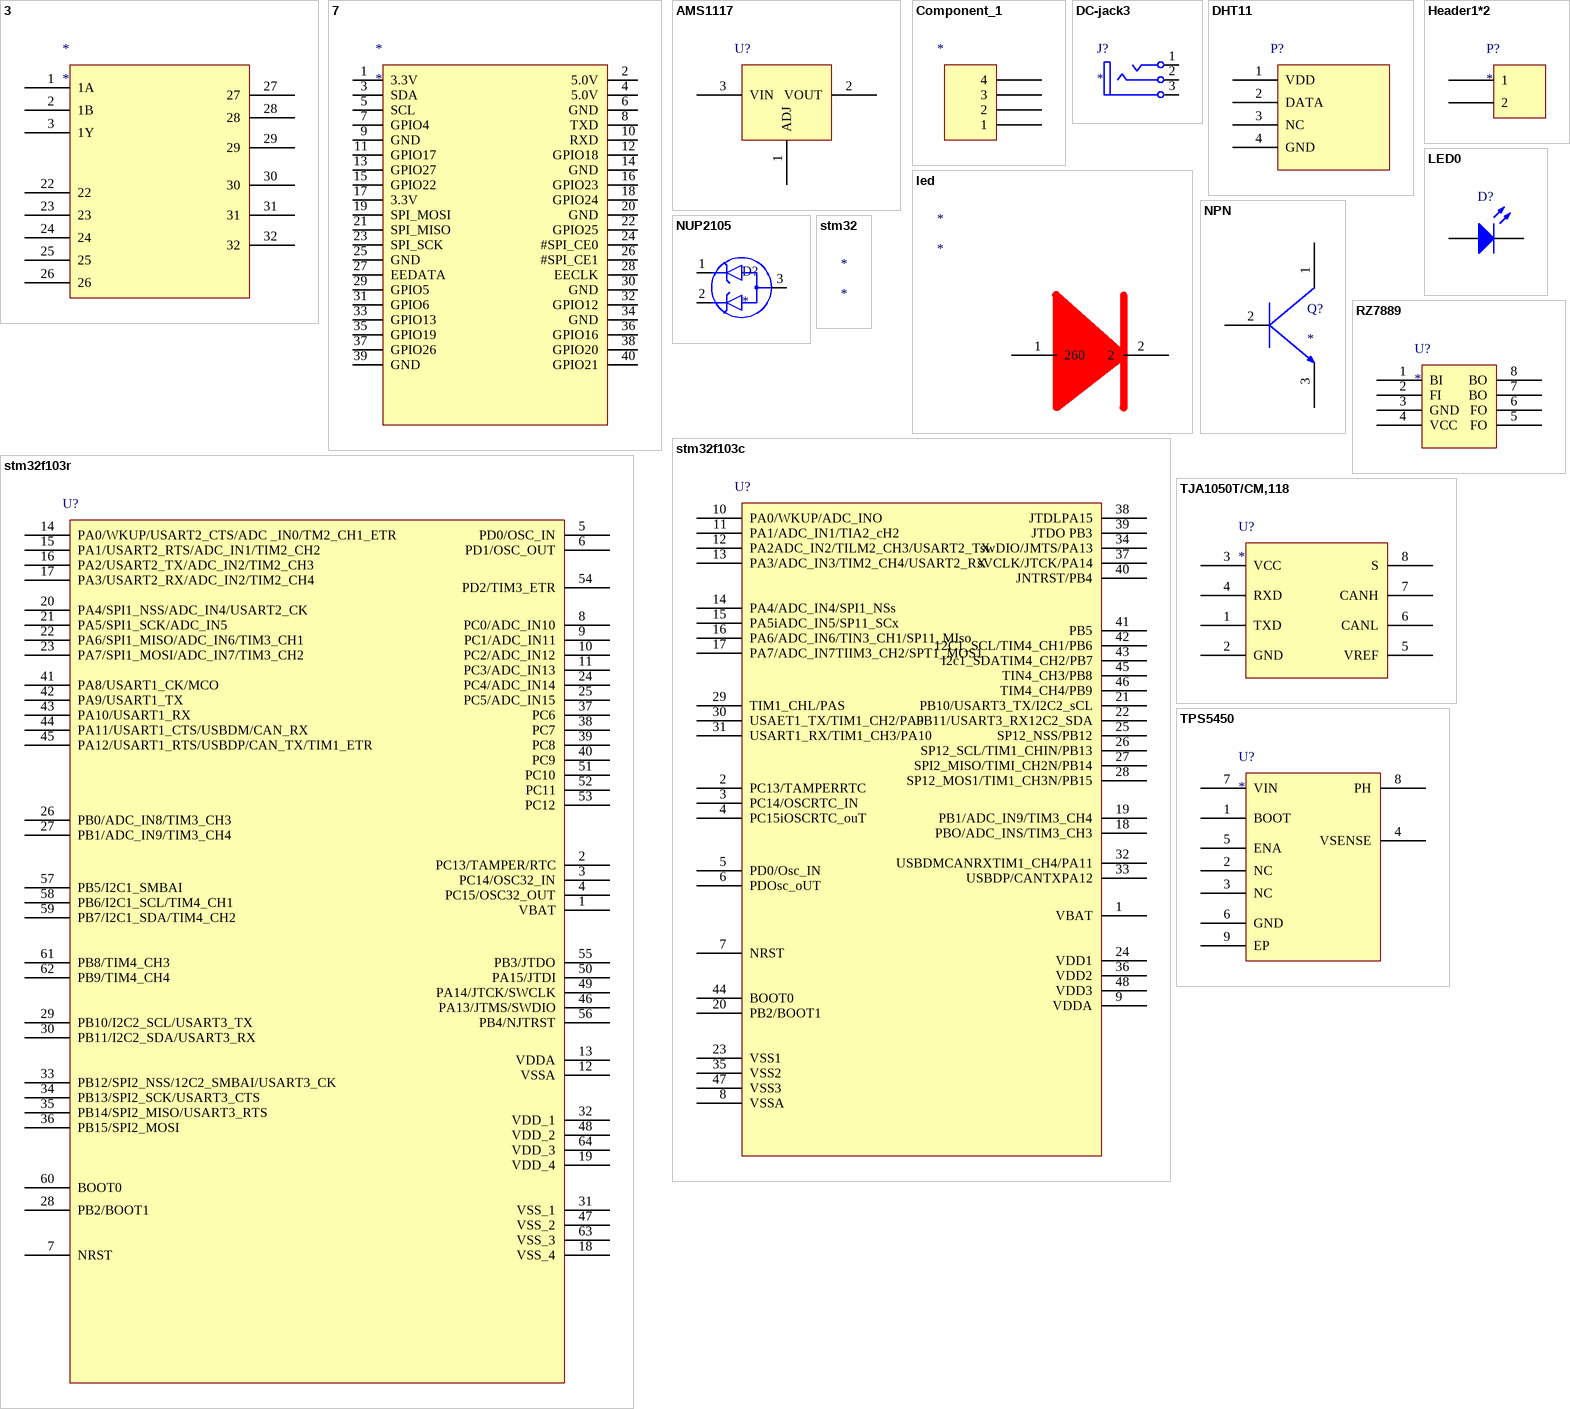
[diagram p0: symbols 3 to TPS5450]
# Altium schematic symbol library MISC82341-24.SchLib: 17 symbols
Pins are listed as number, name and electrical type; pins without a type are passive.


## 3
designator *
pins: 1 1A, 2 1B, 3 1Y, 22, 23, 24, 25, 26, 27, 28, 29, 30, 31, 32

## 7
designator *
pins: 1 3.3V, 2 5.0V, 3 SDA, 4 5.0V, 5 SCL, 6 GND, 7 GPIO4, 8 TXD, 9 GND, 10 RXD, 11 GPIO17, 12 GPIO18, 13 GPIO27, 14 GND, 15 GPIO22, 16 GPIO23, 17 3.3V, 18 GPIO24, 19 SPI_MOSI, 20 GND, 21 SPI_MISO, 22 GPIO25, 23 SPI_SCK, 24 #SPI_CE0, 25 GND, 26 #SPI_CE1, 27 EEDATA, 28 EECLK, 29 GPIO5, 30 GND, 31 GPIO6, 32 GPIO12, 33 GPIO13, 34 GND, 35 GPIO19, 36 GPIO16, 37 GPIO26, 38 GPIO20, 39 GND, 40 GPIO21

## AMS1117
designator U?
footprint SOT-89
pins: 1 ADJ, 2 VOUT, 3 VIN

## Component_1
designator *
pins: ?1 4, ?2 3, ?3 2, ?4 1

## DC-jack3
designator J?
footprint JACK/6-V3
pins: 1 T "Tip/Left Channel/(+)", 2 R "Ring/Right Channel/(-)", 3 S "Sleeve (Ground)"

## DHT11
designator P?
pins: 1 VDD, 2 DATA, 3 NC, 4 GND

## Header1*2
designator P?
footprint HDR1X2
pins: 1, 2

## led
designator *
pins: 1 260, 2

## LED0
designator D?
Typical INFRARED GaAs LED
footprint LED-0 (LED; 2 Leads)
simulation model LED0 (Diode)
pins: 1 A, 2 K

## NPN
designator Q?
footprint QNPN
pins: 1, 2, 3

## NUP2105
designator D?
footprint 123
pins: 1 C1, 2 C2, 3 A

## RZ7889
designator U?
footprint SOP-8
pins: 1 BI, 2 FI, 3 GND, 4 VCC, 5 FO, 6 FO, 7 BO, 8 BO

## stm32
designator *

## stm32f103c
designator U?
pins: 1 VBAT, 2 PC13/TAMPERRTC, 3 PC14/OSCRTC_IN, 4 PC15iOSCRTC_ouT, 5 PD0/Osc_IN, 6 PDOsc_oUT, 7 NRST, 8 VSSA, 9 VDDA, 10 PA0/WKUP/ADC_INO, 11 PA1/ADC_IN1/TIA2_cH2, 12 PA2ADC_IN2/TILM2_CH3/USART2_TX, 13 PA3/ADC_IN3/TIM2_CH4/USART2_RX, 14 PA4/ADC_IN4/SPI1_NSs, 15 PA5iADC_IN5/SP11_SCx, 16 PA6/ADC_IN6/TIN3_CH1/SP11_MIso, 17 PA7/ADC_IN7TIIM3_CH2/SPT1_MOS1, 18 PBO/ADC_INS/TIM3_CH3, 19 PB1/ADC_IN9/TIM3_CH4, 20 PB2/BOOT1, 21 PB10/USART3_TX/I2C2_sCL, 22 PB11/USART3_RX12C2_SDA, 23 VSS1, 24 VDD1, 25 SP12_NSS/PB12, 26 SP12_SCL/TIM1_CHIN/PB13, 27 SPI2_MISO/TIMI_CH2N/PB14, 28 SP12_MOS1/TIM1_CH3N/PB15, 29 TIM1_CHL/PAS, 30 USAET1_TX/TIM1_CH2/PA9, 31 USART1_RX/TIM1_CH3/PA10, 32 USBDMCANRXTIM1_CH4/PA11, 33 USBDP/CANTXPA12, 34 swDIO/JMTS/PA13, 35 VSS2, 36 VDD2, 37 sVCLK/JTCK/PA14, 38 JTDLPA15, 39 JTDO PB3, 40 JNTRST/PB4, 41 PB5, 42 12C1_SCL/TIM4_CH1/PB6, 43 I2c1_SDATIM4_CH2/PB7, 44 BOOT0, 45 TIN4_CH3/PB8, 46 TIM4_CH4/PB9, 47 VSS3, 48 VDD3

## stm32f103r
designator U?
footprint LQFP-64
pins: 1 VBAT, 2 PC13/TAMPER/RTC, 3 PC14/OSC32_IN, 4 PC15/OSC32_OUT, 5 PD0/OSC_IN, 6 PD1/OSC_OUT, 7 NRST, 8 PC0/ADC_IN10, 9 PC1/ADC_IN11, 10 PC2/ADC_IN12, 11 PC3/ADC_IN13, 12 VSSA, 13 VDDA, 14 PA0/WKUP/USART2_CTS/ADC _IN0/TM2_CH1_ETR, 15 PA1/USART2_RTS/ADC_IN1/TIM2_CH2, 16 PA2/USART2_TX/ADC_IN2/TIM2_CH3, 17 PA3/USART2_RX/ADC_IN2/TIM2_CH4, 18 VSS_4, 19 VDD_4, 20 PA4/SPI1_NSS/ADC_IN4/USART2_CK, 21 PA5/SPI1_SCK/ADC_IN5, 22 PA6/SPI1_MISO/ADC_IN6/TIM3_CH1, 23 PA7/SPI1_MOSI/ADC_IN7/TIM3_CH2, 24 PC4/ADC_IN14, 25 PC5/ADC_IN15, 26 PB0/ADC_IN8/TIM3_CH3, 27 PB1/ADC_IN9/TIM3_CH4, 28 PB2/BOOT1, 29 PB10/I2C2_SCL/USART3_TX, 30 PB11/I2C2_SDA/USART3_RX, 31 VSS_1, 32 VDD_1, 33 PB12/SPI2_NSS/12C2_SMBAI/USART3_CK, 34 PB13/SPI2_SCK/USART3_CTS, 35 PB14/SPI2_MISO/USART3_RTS, 36 PB15/SPI2_MOSI, 37 PC6, 38 PC7, 39 PC8, 40 PC9, 41 PA8/USART1_CK/MCO, 42 PA9/USART1_TX, 43 PA10/USART1_RX, 44 PA11/USART1_CTS/USBDM/CAN_RX, 45 PA12/USART1_RTS/USBDP/CAN_TX/TIM1_ETR, 46 PA13/JTMS/SWDIO, 47 VSS_2, 48 VDD_2, 49 PA14/JTCK/SWCLK, 50 PA15/JTDI, 51 PC10, 52 PC11, 53 PC12, 54 PD2/TIM3_ETR, 55 PB3/JTDO, 56 PB4/NJTRST, 57 PB5/I2C1_SMBAI, 58 PB6/I2C1_SCL/TIM4_CH1, 59 PB7/I2C1_SDA/TIM4_CH2, 60 BOOT0, 61 PB8/TIM4_CH3, 62 PB9/TIM4_CH4, 63 VSS_3, 64 VDD_3

## TJA1050T/CM,118
designator U?
footprint SOIC-8
pins: 1 TXD, 2 GND, 3 VCC, 4 RXD, 5 VREF, 6 CANL, 7 CANH, 8 S

## TPS5450
designator U?
footprint SOP-8_L4.9
pins: 1 BOOT, 2 NC, 3 NC, 4 VSENSE, 5 ENA, 6 GND, 7 VIN, 8 PH, 9 EP